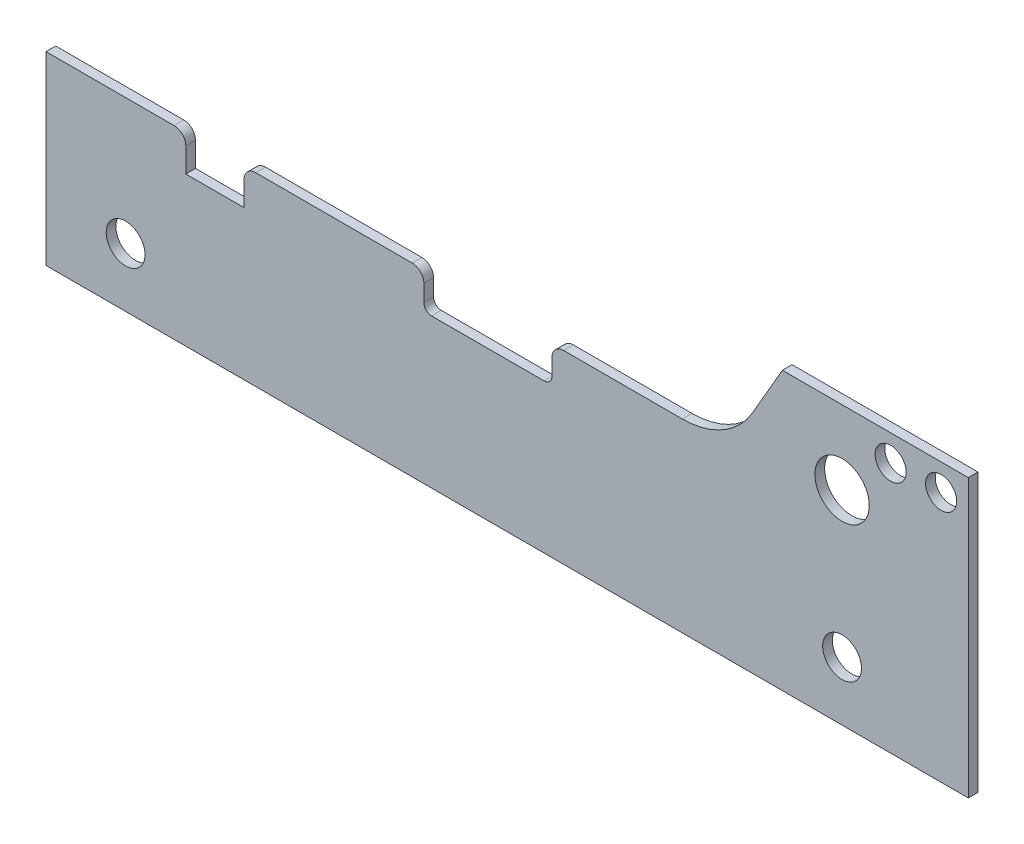
SolidWorks part; units mm, degrees
ref_plane "Front Plane" through (0, 0, 0) normal (0, 0, 1) x (1, 0, 0)
ref_plane "Top Plane" through (0, 0, 0) normal (0, 1, 0) x (1, 0, 0)
ref_plane "Right Plane" through (0, 0, 0) normal (1, 0, 0) x (0, 0, -1)
sketch "Sketch1" plane through (0, 0, 0) normal (0, 0, 1) x (1, 0, 0)
  line L0 (0, 0) -> (0, 477)
  line L1 (0, 477) -> (330, 477)
  line L2 (973, 447) -> (973, 404)
  line L3 (993, 384) -> (1283, 384)
  line L4 (1303, 404) -> (1303, 447)
  line L5 (1333, 477) -> (1638.4131, 477)
  line L6 (1896.2, 714.5) -> (1819.4124, 581.5)
  line L7 (1896.2, 714.5) -> (2375, 714.5)
  line L8 (2375, 714.5) -> (2375, 0)
  line L9 (2375, 0) -> (0, 0)
  line L10 (0, 0) -> (0.3796, -0.3796)
  line L11 (360, 384) -> (360, 447)
  line L12 (510, 384) -> (510, 447)
  line L13 (510, 384) -> (360, 384)
  line L14 (540, 477) -> (943, 477)
  arc A0 (1819.4124, 581.5) -> (1638.4131, 477) centre (1638.4131, 686) cw
  arc A1 (1303, 447) -> (1333, 477) centre (1333, 447) cw
  arc A2 (973, 447) -> (943, 477) centre (943, 447) ccw
  arc A3 (1303, 404) -> (1283, 384) centre (1283, 404) cw
  arc A4 (973, 404) -> (993, 384) centre (993, 404) ccw
  circle A5 centre (205, 151.5) radius 50
  arc A6 (540, 477) -> (510, 447) centre (540, 447) ccw
  circle A7 centre (2050, 151.5) radius 50
  circle A8 centre (2050, 524.5) radius 70
  circle A9 centre (2305, 646.5) radius 40
  circle A10 centre (2175, 646.5) radius 40
  arc A11 (330, 477) -> (360, 447) centre (330, 447) cw
  point P18 (973, 477)
  dimension "D10" = 209
  dimension "D11" = 30
  dimension "D12" = 20
  dimension "D17" = 100
  dimension "D18" = 30
  dimension "D23" = 100
  dimension "D24" = 140
  dimension "D28" = 80
  dimension "D29" = 80
  dimension "D1" = 2375
  dimension "D2" = 973
  dimension "D3" = 477
  dimension "D4" = 384
  dimension "D5" = 150
  dimension "D6" = 477
  dimension "D7" = 714.5
  dimension "D8" = 478.8
  dimension "D9" = 120
  dimension "D13" = 205
  dimension "D14" = 360
  dimension "D15" = 151.5
  dimension "D16" = 384
  dimension "D19" = 151.5
  dimension "D20" = 373
  dimension "D21" = 325
  dimension "D22" = 325
  dimension "D25" = 70
  dimension "D26" = 130
  dimension "D27" = 68
  dimension "D30" = 68
extrude "Boss-Extrude1" add sketch "Sketch1" along normal blind 25
